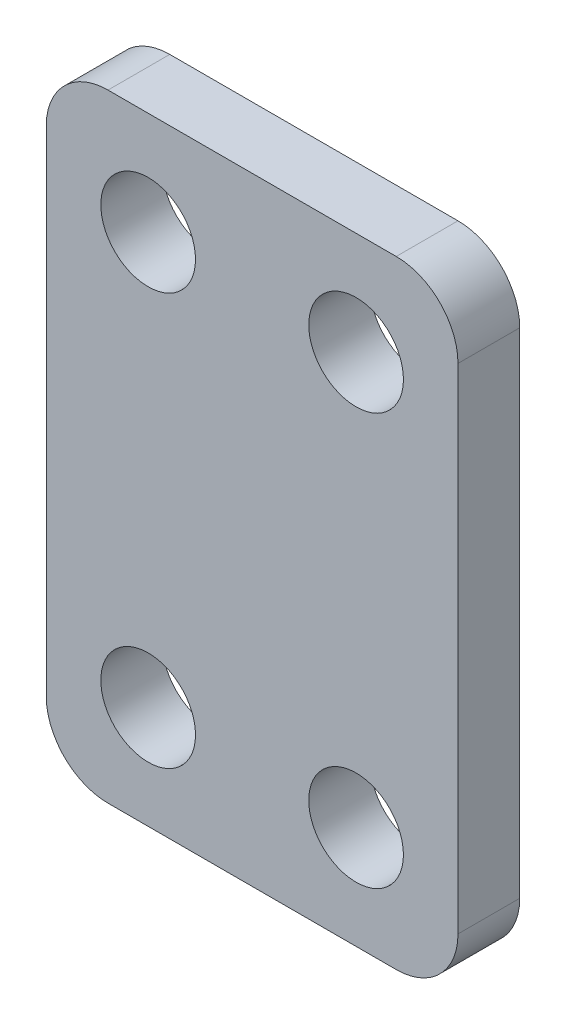
SolidWorks part; units mm, degrees
ref_plane "Front Plane" through (0, 0, 0) normal (0, 0, 1) x (1, 0, 0)
ref_plane "Top Plane" through (0, 0, 0) normal (0, 1, 0) x (1, 0, 0)
ref_plane "Right Plane" through (0, 0, 0) normal (1, 0, 0) x (0, 0, -1)
sketch "Sketch1" plane through (0, 0, 0) normal (0, 0, 1) x (1, 0, 0)
  line L1 (-10, 15) -> (10, 15)
  line L2 (-10, 15) -> (-10, -15)
  line L3 (-10, -15) -> (10, -15)
  line L4 (10, 15) -> (10, -15)
  line L5 (-10, 15) -> (10, -15) construction
  line L6 (-10, -15) -> (10, 15) construction
  point P0 (0, 0)
  dimension "D1" = 20
  dimension "D2" = 30
extrude "Boss-Extrude1" add sketch "Sketch1" along normal blind 3
sketch "Sketch2" plane through (0, 0, 3) normal (0, 0, 1) x (1, 0, 0)
  line L0 (10, 15) -> (-10, 15) construction
  circle A0 centre (-5.05, 10) radius 2.3
  circle A1 centre (5.05, 10) radius 2.3
  circle A2 centre (-5.05, -10) radius 2.3
  circle A3 centre (5.05, -10) radius 2.3
  dimension "D1" = 4.6
  dimension "D2" = 20
  dimension "D3" = 5
  dimension "D4" = 10.1
  dimension "D5" = 5.05
extrude "Cut-Extrude1" cut sketch "Sketch2" against normal blind 3
fillet "Fillet1" radius 3 4 edges at (-10, -15, 1.5) (10, -15, 1.5) (10, 15, 1.5) (-10, 15, 1.5)
